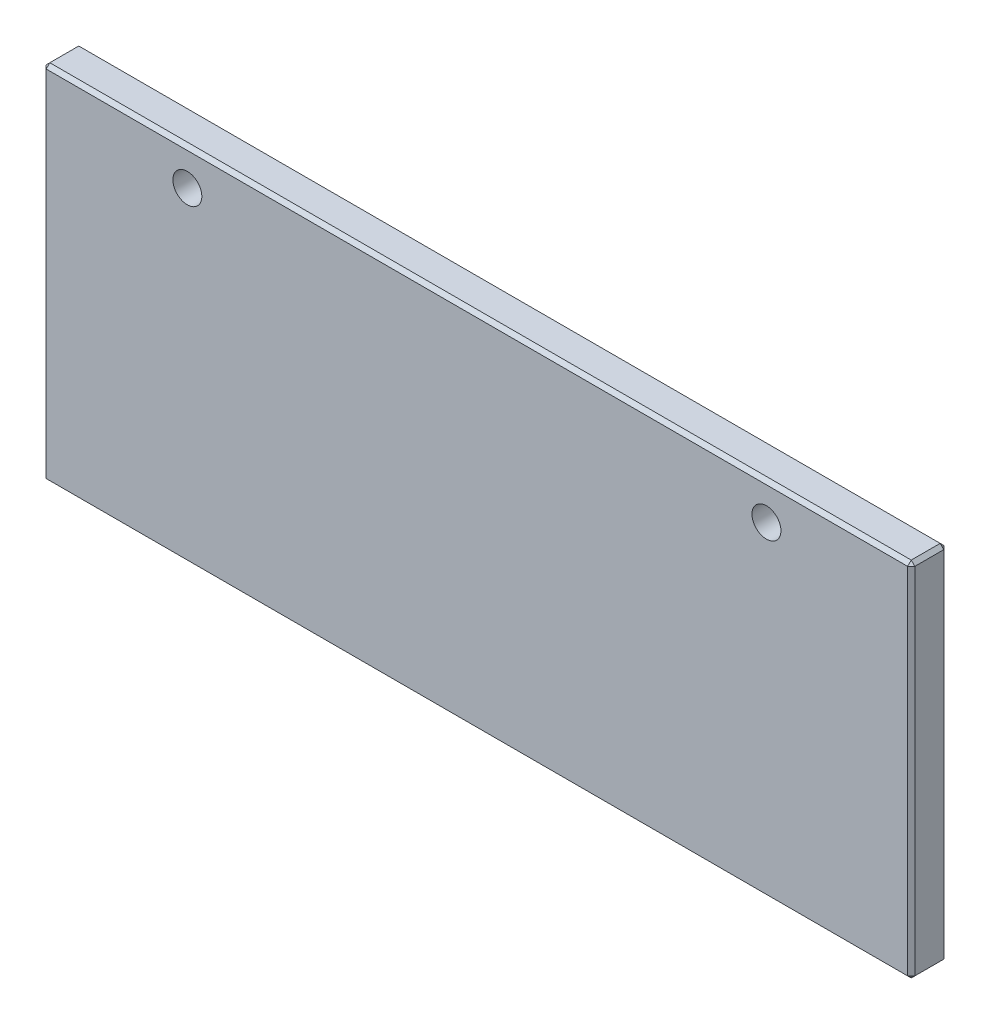
SolidWorks part; units mm, degrees
ref_plane "Front Plane" through (0, 0, 0) normal (0, 0, 1) x (1, 0, 0)
ref_plane "Top Plane" through (0, 0, 0) normal (0, 1, 0) x (1, 0, 0)
ref_plane "Right Plane" through (0, 0, 0) normal (1, 0, 0) x (0, 0, -1)
other "Configuration Table"
sketch "Sketch1" plane through (0, 0, 0) normal (0, 0, 1) x (1, 0, 0)
  line L1 (0, 0) -> (120, 0)
  line L2 (0, 0) -> (0, 50)
  line L3 (0, 50) -> (120, 50)
  line L4 (120, 0) -> (120, 50)
  dimension "D1" = 120
  dimension "D2" = 50
extrude "Boss-Extrude1" add sketch "Sketch1" along normal blind 5
sketch "Sketch2" plane through (0, 0, 5) normal (0, 0, 1) x (1, 0, 0)
  line L0 (120, 50) -> (0, 50) construction
  line L1 (0, 50) -> (0, 0) construction
  line L3 (120, 0) -> (120, 50) construction
  point P0 (20, 45)
  point P1 (100, 45)
  dimension "D1" = 80
  dimension "D2" = 5
  dimension "D3" = 20
  dimension "D4" = 20
hole_wizard "Ø4.0mm dowel hole1" positions "Sketch2" profile "Sketch3" hole size "Ø4.0" standard "GB"
sketch "Sketch3" plane through (20, 45, 5) normal (1, 0, 0) x (0, -1, 0)
  line L0 (0, 0) -> (0, 13.2017)
  line L1 (0, 13.2017) -> (2, 12)
  line L2 (2, 12) -> (2, 0)
  line L5 (2, 0) -> (0, 0)
  line L10 (0, 13.2017) -> (-2, 12) construction
  line L11 (0, -6.35) -> (0, 107.95) construction
  dimension "孔直径" = 4
  dimension "孔深度" = 12
  dimension "导头角度" = 118
chamfer "Chamfer1" distance 0.5 12 edges at (120, 25, 5) (120, 25, 0) (60, 0, 5) (120, 0, 2.5) (60, 0, 0) (120, 50, 2.5) (60, 50, 5) (60, 50, 0) (0, 50, 2.5) (0, 25, 5) (0, 0, 2.5) (0, 25, 0)
